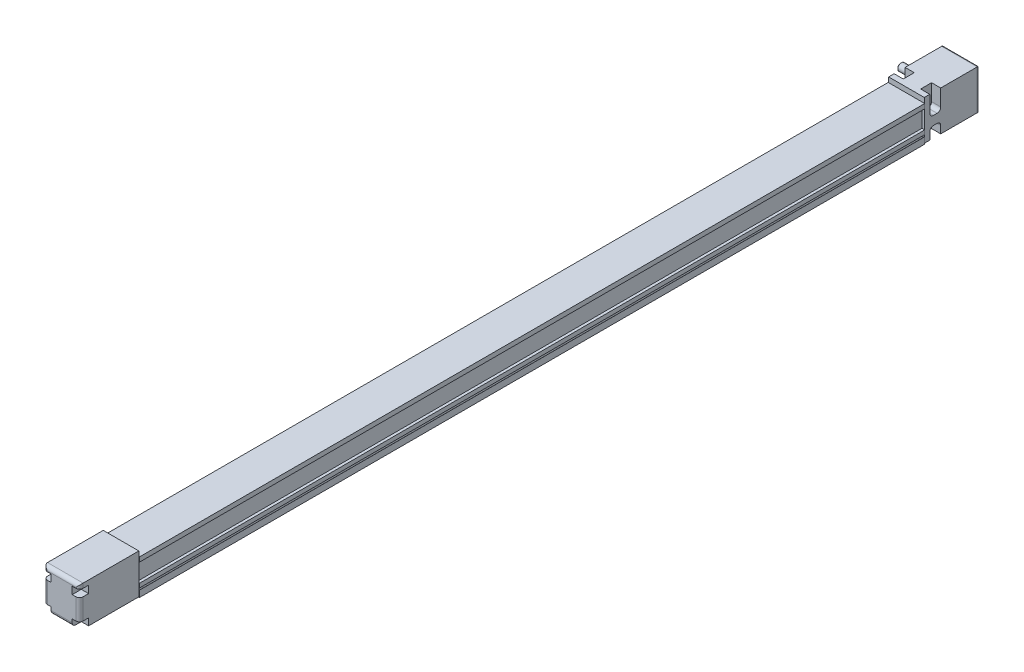
SolidWorks part; units mm, degrees
ref_plane "前视" through (0, 0, 0) normal (0, 0, 1) x (1, 0, 0)
ref_plane "上视" through (0, 0, 0) normal (0, 1, 0) x (1, 0, 0)
ref_plane "右视" through (0, 0, 0) normal (1, 0, 0) x (0, 0, -1)
sketch "草图1" plane through (0, 0, 0) normal (0, 0, 1) x (1, 0, 0)
  line L0 (20, 38.5578) -> (20, -6.3921) construction
  line L1 (0, 0) -> (40, 0)
  line L2 (0, 0) -> (0, 7)
  line L3 (0, 38.5578) -> (40, 38.5578)
  line L4 (40, 9.0578) -> (40, 13.5578)
  line L5 (0, 7) -> (2, 5.0578)
  line L6 (2, 5.0578) -> (2, 9.0578)
  line L7 (2, 9.0578) -> (0, 9.0578)
  line L8 (0, 13.5578) -> (3, 13.5578)
  line L9 (3, 13.5578) -> (3, 33.5578)
  line L10 (3, 33.5578) -> (0, 33.5578)
  line L11 (0, 33.5578) -> (0, 38.5578)
  line L12 (0, 9.0578) -> (0, 13.5578)
  line L13 (40, 33.5578) -> (40, 38.5578)
  line L14 (37, 33.5578) -> (40, 33.5578)
  line L15 (37, 13.5578) -> (37, 33.5578)
  line L16 (40, 13.5578) -> (37, 13.5578)
  line L17 (38, 9.0578) -> (40, 9.0578)
  line L18 (38, 5.0578) -> (38, 9.0578)
  line L19 (40, 7) -> (38, 5.0578)
  line L20 (40, 0) -> (40, 7)
  point P23 (20, 0)
  dimension "D1" = 5
  dimension "D2" = 20
  dimension "D3" = 4.5
  dimension "D4" = 3
  dimension "D5" = 2
  dimension "D6" = 4
  dimension "D7" = 7
  dimension "D8" = 20
extrude "基体-拉伸" add sketch "草图1" along normal blind 860
sketch "草图2" plane through (0, 0, 860) normal (0, 0, 1) x (1, 0, 0)
  line L0 (0, 38.5578) -> (0, 33.5578) construction
  line L1 (0.5, 0.5) -> (39.5, 0.5)
  line L2 (0.5, 0.5) -> (0.5, 44.0578)
  line L3 (0.5, 44.0578) -> (39.5, 44.0578)
  line L4 (39.5, 0.5) -> (39.5, 44.0578)
  line L5 (40, 33.5578) -> (40, 38.5578) construction
  line L6 (40, 38.5578) -> (0, 38.5578) construction
  line L7 (0, 0) -> (40, 0) construction
  dimension "D1" = 0.5
  dimension "D2" = 0.5
  dimension "D3" = 5.5
  dimension "D4" = 0.5
extrude "凸台-拉伸1" add sketch "草图2" along normal blind 65
fillet "圆角2" radius 4 4 edges at (0.5, 22.2789, 925) (20, 0.5, 925) (39.5, 22.2789, 925) (20, 44.0578, 925)
sketch "草图3" plane through (0, 0, 925) normal (0, 0, 1) x (1, 0, 0)
  line L2 (0.5, 39.134) -> (0.5, 31.134)
  line L3 (8.5, 31.134) -> (0.5, 31.134)
  line L4 (8.5, 39.134) -> (8.5, 31.134)
  line L6 (20, 0.5) -> (20, 44.5578) construction
  line L7 (39.5, 0.5) -> (0.5, 0.5) construction
  line L8 (8.5, 39.134) -> (0.5, 39.134)
  line L9 (31.5, 8.134) -> (39.5, 8.134)
  line L10 (31.5, 8.134) -> (31.5, 0.134)
  line L11 (31.5, 0.134) -> (39.5, 0.134)
  line L12 (39.5, 8.134) -> (39.5, 0.134)
  line L13 (31.5, 39.134) -> (39.5, 39.134)
  line L14 (31.5, 39.134) -> (31.5, 31.134)
  line L15 (31.5, 31.134) -> (39.5, 31.134)
  line L16 (39.5, 39.134) -> (39.5, 31.134)
  line L17 (0.5, 8.134) -> (0.5, 0.134)
  line L18 (8.5, 0.134) -> (0.5, 0.134)
  line L19 (8.5, 8.134) -> (8.5, 0.134)
  line L20 (8.5, 8.134) -> (0.5, 8.134)
  dimension "D1" = 8
  dimension "D2" = 8
extrude "切除-拉伸1" cut sketch "草图3" against normal blind 10
sketch "草图4" plane through (0, 0, 0) normal (0, 0, -1) x (-1, 0, 0)
  line L0 (0, 38.5578) -> (0, 33.5578) construction
  line L1 (-39.5, 0.5) -> (-0.5, 0.5)
  line L2 (-39.5, 0.5) -> (-39.5, 44.0578)
  line L3 (-39.5, 44.0578) -> (-0.5, 44.0578)
  line L4 (-0.5, 0.5) -> (-0.5, 44.0578)
  line L5 (-40, 9.0578) -> (-40, 13.5578) construction
  line L7 (0, 0) -> (-40, 0) construction
  line L8 (-40, 38.5578) -> (0, 38.5578) construction
  dimension "D1" = 0.5
  dimension "D2" = 0.5
  dimension "D3" = 0.5
  dimension "D4" = 5.5
extrude "凸台-拉伸3" add sketch "草图4" along normal blind 60
fillet "圆角4" radius 2 4 edges at (39.5, 22.2789, -60) (20, 0.5, -60) (0.5, 22.2789, -60) (20, 44.0578, -60)
sketch "草图5" plane through (0.5, 0, 0) normal (-1, 0, 0) x (0, 0, 1)
  line L0 (-58, 44.0578) -> (0, 44.0578) construction
  line L1 (-18, 44.0578) -> (-6, 44.0578)
  line L2 (-18, 44.0578) -> (-18, 26.0578)
  line L3 (-14, 22.0578) -> (-10, 22.0578)
  line L4 (-6, 44.0578) -> (-6, 26.0578)
  line L5 (0, 38.5578) -> (0, 44.0578) construction
  line L6 (-58, 0.5) -> (0, 0.5) construction
  line L7 (-14, 12.5) -> (-10, 12.5)
  line L8 (-18, 8.5) -> (-18, 0.5)
  line L9 (-18, 0.5) -> (-6, 0.5)
  line L10 (-6, 8.5) -> (-6, 0.5)
  arc A0 (-10, 22.0578) -> (-6, 26.0578) centre (-10, 26.0578) ccw
  arc A1 (-14, 22.0578) -> (-18, 26.0578) centre (-14, 26.0578) cw
  arc A2 (-14, 12.5) -> (-18, 8.5) centre (-14, 8.5) ccw
  arc A3 (-6, 8.5) -> (-10, 12.5) centre (-10, 8.5) ccw
  point P10 (-6, 22.0578)
  point P21 (-18, 12.5)
  dimension "D4" = 4
  dimension "D6" = 4
  dimension "D1" = 6
  dimension "D2" = 12
  dimension "D3" = 22
  dimension "D5" = 12
extrude "切除-拉伸2" cut sketch "草图5" against normal blind 10
sketch "草图7" plane through (39.5, 0, 0) normal (1, 0, 0) x (0, 0, -1)
  line L0 (58, 44.0578) -> (0, 44.0578) construction
  line L1 (6, 44.0578) -> (18, 44.0578)
  line L2 (6, 44.0578) -> (6, 26.0578)
  line L3 (10, 22.0578) -> (14, 22.0578)
  line L4 (18, 44.0578) -> (18, 26.0578)
  line L5 (0, 44.0578) -> (0, 38.5578) construction
  line L6 (58, 0.5) -> (0, 0.5) construction
  line L7 (10, 12.5) -> (14, 12.5)
  line L8 (6, 8.5) -> (6, 0.5)
  line L9 (6, 0.5) -> (18, 0.5)
  line L10 (18, 8.5) -> (18, 0.5)
  line L11 (0, 0) -> (0, 7) construction
  arc A0 (14, 12.5) -> (18, 8.5) centre (14, 8.5) cw
  arc A1 (10, 12.5) -> (6, 8.5) centre (10, 8.5) ccw
  arc A2 (6, 26.0578) -> (10, 22.0578) centre (10, 26.0578) ccw
  arc A3 (14, 22.0578) -> (18, 26.0578) centre (14, 26.0578) ccw
  point P16 (18, 12.5)
  point P23 (18, 22.0578)
  dimension "D5" = 4
  dimension "D1" = 22
  dimension "D2" = 6
  dimension "D3" = 12
  dimension "D4" = 12
  dimension "D6" = 6
  dimension "D7" = 12
extrude "切除-拉伸3" cut sketch "草图7" against normal blind 10
hole_wizard "M4 螺纹孔1" positions "草图12" profile "草图11" tap size "M4" standard "GB"
sketch "草图12" plane through (0.5, 0, 0) normal (-1, 0, 0) x (0, 0, 1)
  line L1 (-54, 38.5578) -> (-22, 38.5578) construction
  line L2 (-54, 38.5578) -> (-54, 6.5578) construction
  line L3 (-54, 6.5578) -> (-22, 6.5578) construction
  line L4 (-22, 38.5578) -> (-22, 6.5578) construction
  line L5 (-60, 2.5) -> (-60, 42.0578) construction
  line L6 (-58, 44.0578) -> (-18, 44.0578) construction
  point P0 (-22, 6.5578)
  point P1 (-54, 6.5578)
  point P3 (-22, 38.5578)
  point P5 (-54, 38.5578)
  dimension "D1" = 32
  dimension "D2" = 32
  dimension "D3" = 6
  dimension "D4" = 5.5
sketch "草图11" plane through (0.5, 6.5578, -22) normal (0, 1, 0) x (0, 0, 1)
  line L0 (0, 0) -> (0, 11.0914)
  line L1 (0, 11.0914) -> (1.65, 10.1)
  line L2 (1.65, 10.1) -> (1.65, 0)
  line L5 (1.65, 0) -> (0, 0)
  line L10 (0, 11.0914) -> (-1.65, 10.1) construction
  line L11 (0, -6.35) -> (0, 107.95) construction
  dimension "螺纹孔钻头直径" = 3.3
  dimension "螺纹孔钻头深度" = 10.1
  dimension "导头角度" = 118
cosmetic thread "孔螺蚊线1" parameters "D1"=8, "D2"=4
cosmetic thread "孔螺蚊线2" parameters "D1"=8, "D2"=4
cosmetic thread "孔螺蚊线3" parameters "D1"=8, "D2"=4
cosmetic thread "孔螺蚊线4" parameters "D1"=8, "D2"=4
sketch "草图13" plane through (0.5, 0, 0) normal (-1, 0, 0) x (0, 0, 1)
  circle A0 centre (-38, 22.5578) radius 22.6274 construction
  circle A1 centre (-38, 22.5578) radius 18.5
  dimension "D1" = 37
extrude "切除-拉伸4" cut sketch "草图13" against normal blind 3
sketch "草图14" plane through (3.5, 0, 0) normal (-1, 0, 0) x (0, 0, 1)
  circle A0 centre (-38, 22.5578) radius 4
  dimension "D1" = 8
extrude "凸台-拉伸5" add sketch "草图14" along normal blind 28
chamfer "倒角1" distance 1 angle 45 1 edges at (-24.5, 22.5578, -34)
